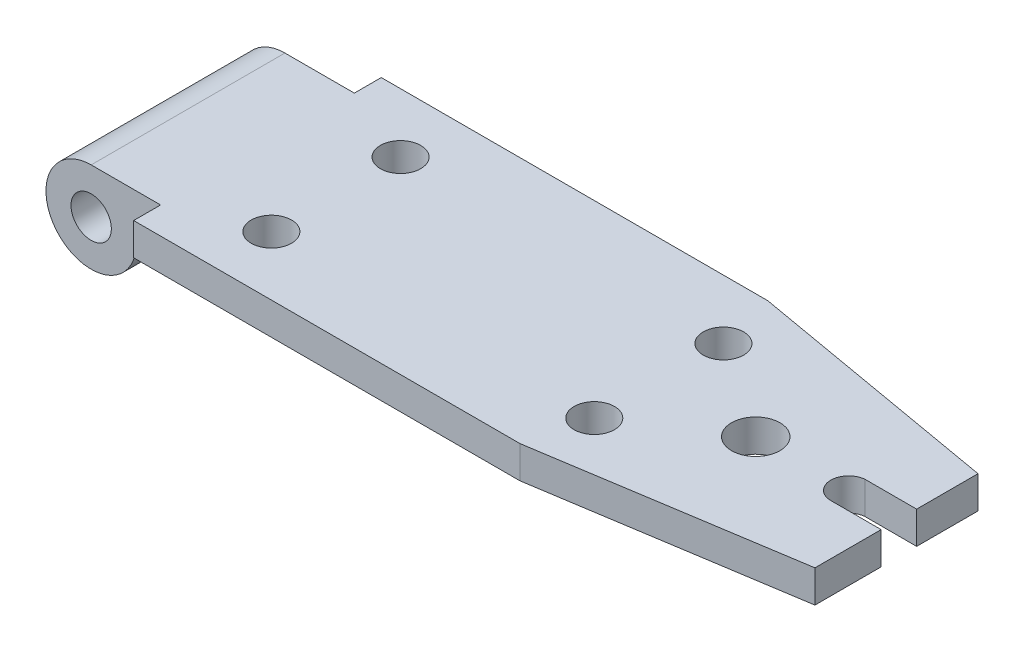
from build123d import *

# Parameters (mm, degrees)
SKETCH1_R           = 12.5
SKETCH1_R_2         = 15
BOSS_EXTRUDE1_DEPTH = 20
SKETCH2_R           = 12.5
BOSS_EXTRUDE3_DEPTH = 60


with BuildPart() as part:
    # Sketch1 → Boss-Extrude1 (new body)
    with BuildSketch(Plane(origin=(0, 0, 0), x_dir=(1, 0, 0), z_dir=(0, 1, 0))):
        with BuildLine():
            Line((-156.766665721, -76.687206232), (82.57489949, -76.687206232))
            Line((82.57489949, -76.687206232), (240.511245974, -51.99105161))
            Line((240.511245974, -51.99105161), (240.511245974, -11))
            Line((240.511245974, -11), (208.511245974, -11))
            ThreePointArc((208.511245974, -11), (198.376578208, 0), (208.511245974, 11))
            Line((208.511245974, 11), (240.511245974, 11))
            Line((240.511245974, 11), (240.511245974, 49))
            Line((240.511245974, 49), (82.57489949, 76.687206232))
            Line((82.57489949, 76.687206232), (-156.766665721, 76.687206232))
            Line((-156.766665721, 76.687206232), (-156.766665721, 60))
            Line((-156.766665721, 60), (-171.766665721, 60))
            Line((-171.766665721, 60), (-171.766665721, -60))
            Line((-171.766665721, -60), (-156.766665721, -60))
            Line((-156.766665721, -60), (-156.766665721, -76.687206232))
        make_face()
        with Locations(Location((-108.150428542, 40, 0), (0, 0, 270))):
            Circle(SKETCH1_R, mode=Mode.SUBTRACT)
        with Locations(Location((-108.150428542, -40, 0), (0, 0, 270))):
            Circle(SKETCH1_R, mode=Mode.SUBTRACT)
        with Locations(Location((91.849571458, 40, 0), (0, 0, 270))):
            Circle(SKETCH1_R, mode=Mode.SUBTRACT)
        with Locations(Location((91.849571458, -40, 0), (0, 0, 270))):
            Circle(SKETCH1_R, mode=Mode.SUBTRACT)
        with Locations(Location((151.849571458, 0, 0), (0, 0, 270))):
            Circle(SKETCH1_R_2, mode=Mode.SUBTRACT)
    extrude(amount=BOSS_EXTRUDE1_DEPTH)

    # Sketch2 → Boss-Extrude3 (add, symmetric)
    with BuildSketch(Plane.XY):
        with BuildLine():
            Line((-199.766665721, 20), (-171.766665721, 20))
            Line((-171.766665721, 20), (-171.766665721, -8))
            ThreePointArc((-171.766665721, -8), (-219.565655594, -27.798989873), (-199.766665721, 20))
        make_face()
        with Locations((-199.766665721, -8)):
            Circle(SKETCH2_R, mode=Mode.SUBTRACT)
    extrude(amount=BOSS_EXTRUDE3_DEPTH, both=True)


solid = part.part
